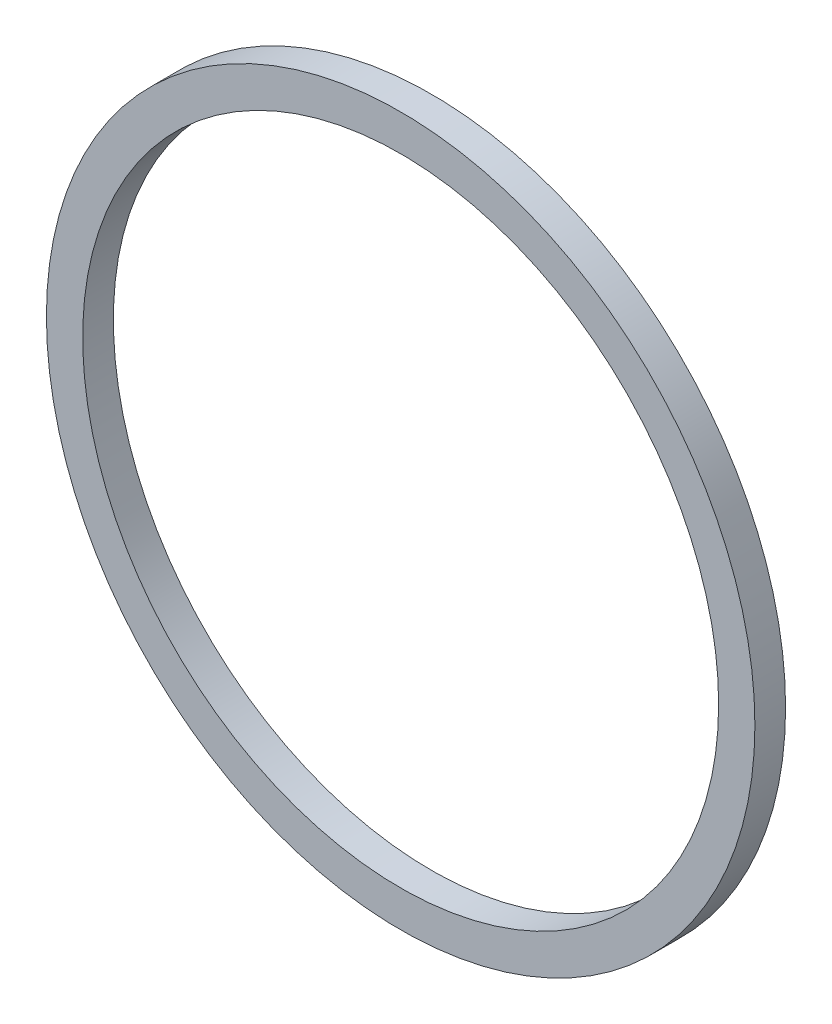
from build123d import *

# Parameters (mm, degrees)
SKETCH1_R           = 63.5
SKETCH1_R_2         = 57
BOSS_EXTRUDE1_DEPTH = 5.5


with BuildPart() as part:
    # Sketch1 → Boss-Extrude1 (new body)
    with BuildSketch(Plane.XY):
        Circle(SKETCH1_R)
        Circle(SKETCH1_R_2, mode=Mode.SUBTRACT)
    extrude(amount=BOSS_EXTRUDE1_DEPTH)


solid = part.part
